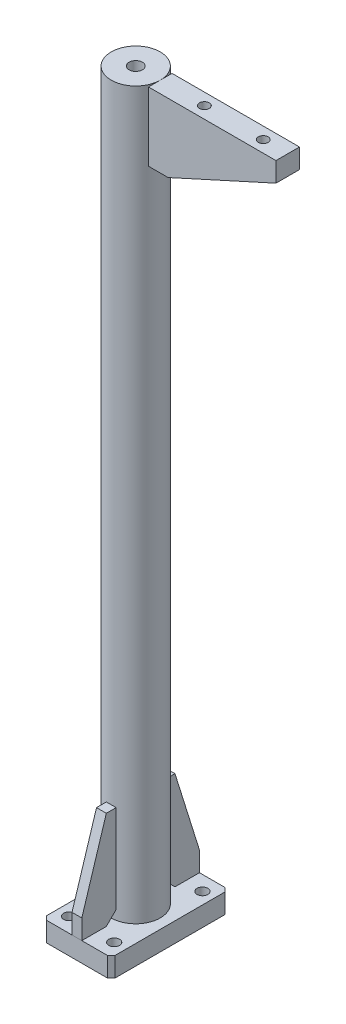
from build123d import *

# Parameters (mm, degrees)
SKETCH_1_R                  = 12.5
EXTRUDE_1_DEPTH             = 370
SKETCH_2_W                  = 35
SKETCH_2_H                  = 60
EXTRUDE_2_DEPTH             = 10
EXTRUDE_3_DEPTH             = 6
HOLE_WIZARD_M6_1_AT_2_COUNT = 2
HOLE_WIZARD_M6_1_AT_2_PITCH = 30
EXTRUDE_4_DEPTH             = 2.5
EXTRUDE_4_2_DEPTH           = 2.5
HOLE_WIZARD_M5_1_AT_2_COUNT = 2
HOLE_WIZARD_M5_1_AT_2_PITCH = 23
HOLE_WIZARD_M5_1_AT_3_COUNT = 2
HOLE_WIZARD_M5_1_AT_3_PITCH = 50.537115074
HOLE_WIZARD_M5_1_AT_4_COUNT = 2
HOLE_WIZARD_M5_1_AT_4_PITCH = 45
CHAMFER_1_SIZE              = 2


with BuildPart() as part:
    # 草图1 → 凸台-拉伸1 (new body)
    with BuildSketch(Plane(origin=(0, 0, 0), x_dir=(1, 0, 0), z_dir=(0, 1, 0))):
        with Locations(Location((0, 0, 0), (0, 0, 270))):
            Circle(SKETCH_1_R)
    extrude(amount=EXTRUDE_1_DEPTH)

    # 草图5 → M8 螺纹孔1 (revolve, cut)
    with BuildSketch(Plane(origin=(0, 370, 0), x_dir=(0, 0, 1), z_dir=(1, 0, 0))):
        Polygon((0, 0), (0, 21.792926105), (3.4, 19.75), (3.4, 0), align=None)
    revolve(axis=Axis((0, 376.35, 0), (0, -1, 0)), mode=Mode.SUBTRACT)


with BuildPart() as body_2:
    # 草图2 → 凸台-拉伸2 (new body)
    with BuildSketch(Plane.XZ):
        Rectangle(SKETCH_2_W, SKETCH_2_H)
    extrude(amount=EXTRUDE_2_DEPTH)

    # 草图10 → M5 间隙孔1 (revolve, cut)
    with BuildSketch(Plane(origin=(11.5, -10, -22.5), x_dir=(0, 0, -1), z_dir=(1, 0, 0))):
        Polygon((0, 0), (0, 16.652366702), (2.75, 15), (2.75, 0), align=None)
    hole_wizard_m5_1 = revolve(axis=Axis((11.5, -16.35, -22.5), (0, 1, 0)), mode=Mode.SUBTRACT)

    # M5 间隙孔1 at 2: M5 间隙孔1 ×2
    with Locations(*[(-i * HOLE_WIZARD_M5_1_AT_2_PITCH, 0, 0) for i in range(1, HOLE_WIZARD_M5_1_AT_2_COUNT)]):
        add(hole_wizard_m5_1, mode=Mode.SUBTRACT)

    # M5 间隙孔1 at 3: M5 间隙孔1 ×2
    with Locations(*[Vector(-0.45511105978910793, 0, 0.8904346821960806) * (i * HOLE_WIZARD_M5_1_AT_3_PITCH) for i in range(1, HOLE_WIZARD_M5_1_AT_3_COUNT)]):
        add(hole_wizard_m5_1, mode=Mode.SUBTRACT)

    # M5 间隙孔1 at 4: M5 间隙孔1 ×2
    with Locations(*[(0, 0, i * HOLE_WIZARD_M5_1_AT_4_PITCH) for i in range(1, HOLE_WIZARD_M5_1_AT_4_COUNT)]):
        add(hole_wizard_m5_1, mode=Mode.SUBTRACT)

    # 倒角1
    chamfer_1_edges = [body_2.edges().sort_by_distance(p)[0] for p in [
        (-17.5, -5, 30),
        (17.5, -5, 30),
        (17.5, -5, -30),
        (-17.5, -5, -30),
    ]]
    chamfer(chamfer_1_edges, length=CHAMFER_1_SIZE)


with BuildPart() as body_3:
    # 草图3 → 凸台-拉伸3 (new, symmetric)
    with BuildSketch(Plane.XY):
        Polygon((12.5, 370), (77.5, 370), (77.5, 360), (22.5, 335), (12.5, 335), align=None)
    extrude(amount=EXTRUDE_3_DEPTH, both=True)

    # 草图7 → M6 螺纹孔1 (revolve, cut)
    with BuildSketch(Plane(origin=(35, 370, 0), x_dir=(0, 0, 1), z_dir=(1, 0, 0))):
        Polygon((0, 0), (0, 16.502151548), (2.5, 15), (2.5, 0), align=None)
    hole_wizard_m6_1 = revolve(axis=Axis((35, 376.35, 0), (0, -1, 0)), mode=Mode.SUBTRACT)

    # M6 螺纹孔1 at 2: M6 螺纹孔1 ×2
    with Locations(*[(i * HOLE_WIZARD_M6_1_AT_2_PITCH, 0, 0) for i in range(1, HOLE_WIZARD_M6_1_AT_2_COUNT)]):
        add(hole_wizard_m6_1, mode=Mode.SUBTRACT)


with BuildPart() as body_4:
    # 草图8 → 凸台-拉伸4 (new, symmetric)
    with BuildSketch(Plane(origin=(0, 0, 0), x_dir=(0, 0, -1), z_dir=(1, 0, 0))):
        Polygon((30, 0), (30, 10), (17.5, 50), (12.5, 50), (12.5, 5), (17.5, 0), align=None)
    extrude(amount=EXTRUDE_4_DEPTH, both=True)


with BuildPart() as body_5:
    # 草图8 → Extrude 4 2 (new, symmetric)
    with BuildSketch(Plane(origin=(0, 0, 0), x_dir=(0, 0, -1), z_dir=(1, 0, 0))):
        Polygon((-12.5, 5), (-17.5, 0), (-30, 0), (-30, 10), (-17.5, 50), (-12.5, 50), align=None)
    extrude(amount=EXTRUDE_4_2_DEPTH, both=True)


solid = Compound([part.part, body_2.part, body_3.part, body_4.part, body_5.part])
